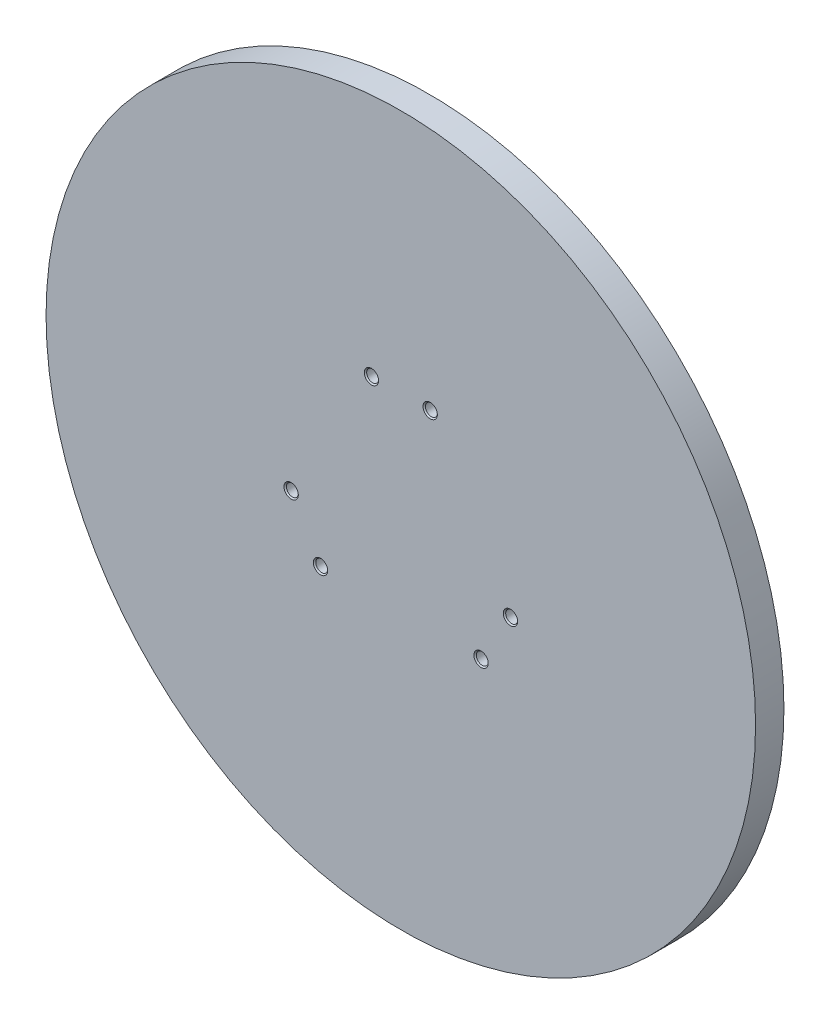
SolidWorks part; units mm, degrees
material "1.7005 (45Cr2)"
ref_plane "前视基准面" through (0, 0, 0) normal (0, 0, 1) x (1, 0, 0)
ref_plane "上视基准面" through (0, 0, 0) normal (0, 1, 0) x (1, 0, 0)
ref_plane "右视基准面" through (0, 0, 0) normal (1, 0, 0) x (0, 0, -1)
sketch "草图1" plane through (0, 0, 0) normal (0, 0, 1) x (1, 0, 0)
  circle A0 centre (0, 0) radius 125
  dimension "D1" = 250
extrude "凸台-拉伸1" add sketch "草图1" along normal blind 10
sketch "草图2" plane through (0, 0, 10) normal (0, 0, 1) x (1, 0, 0)
  line L0 (0, 0) -> (0, 40) construction
  line L1 (0, 0) -> (10.3528, 38.637) construction
  line L2 (0, 0) -> (-10.3528, 38.637) construction
  dimension "D1" = 40
  dimension "D2" = 15
  dimension "D3" = 15
hole_wizard "M5x0.8 螺纹孔1" positions "3D草图1" profile "草图4" tap size "M5x0.8" standard "BSI"
sketch3d "3D草图1"
  point P0 (10.3528, 38.637, 10)
  point P3 (-10.3528, 38.637, 10)
cosmetic thread "孔螺蚊线1" parameters "D1"=10, "D2"=5
cosmetic thread "孔螺蚊线2" parameters "D1"=10, "D2"=5
sketch "草图4" plane through (10.3528, 38.637, 10) normal (1, 0, 0) x (0, -1, 0)
  line L0 (0, 0) -> (0, 13.6618)
  line L1 (0, 13.6618) -> (2.1, 12.4)
  line L2 (2.1, 12.4) -> (2.1, 0.425)
  line L3 (2.1, 0.425) -> (2.525, 0)
  line L5 (2.525, 0) -> (0, 0)
  line L6 (-2.1, 0.425) -> (-2.525, 0) construction
  line L10 (0, 13.6618) -> (-2.1, 12.4) construction
  line L11 (0, -6.35) -> (0, 107.95) construction
  dimension "螺纹孔钻头直径" = 4.2
  dimension "螺纹孔钻头深度" = 12.4
  dimension "近端锥形沉头孔直径" = 5.05
  dimension "近端锥形沉头孔角度" = 90
  dimension "导头角度" = 118
pattern_circular "阵列(圆周)1" count 3 over 360 about axis through (0, 0, 0) along (0, 0, 1) of "M5x0.8 螺纹孔1"
cosmetic thread "孔螺蚊线3" parameters "D1"=10, "D2"=5
cosmetic thread "孔螺蚊线4" parameters "D1"=10, "D2"=5
cosmetic thread "孔螺蚊线5" parameters "D1"=10, "D2"=5
cosmetic thread "孔螺蚊线6" parameters "D1"=10, "D2"=5
